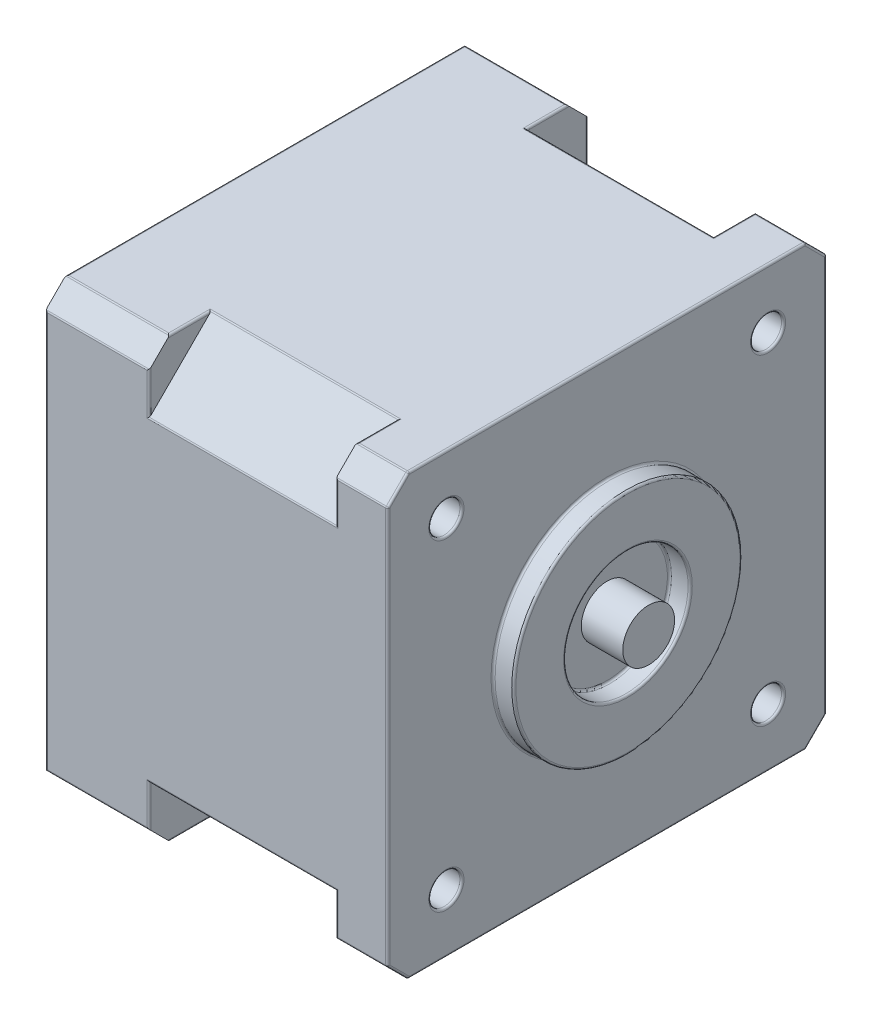
SolidWorks part; units mm, degrees
ref_plane "Front Plane" through (0, 0, 0) normal (0, 0, 1) x (1, 0, 0)
ref_plane "Top Plane" through (0, 0, 0) normal (0, 1, 0) x (1, 0, 0)
ref_plane "Right Plane" through (0, 0, 0) normal (1, 0, 0) x (0, 0, -1)
ref_plane "Plane1" through (16.5, 0, 0) normal (1, 0, 0) x (0, 0, -1)
sketch "Sketch1" plane through (16.5, 0, 0) normal (1, 0, 0) x (0, 0, -1)
  line L0 (-21.15, 19.15) -> (-21.15, -19.15)
  line L1 (-21.15, -19.15) -> (-19.15, -21.15)
  line L2 (-19.15, -21.15) -> (19.15, -21.15)
  line L3 (19.15, -21.15) -> (21.15, -19.15)
  line L4 (21.15, -19.15) -> (21.15, 19.15)
  line L5 (21.15, 19.15) -> (19.15, 21.15)
  line L6 (19.15, 21.15) -> (-19.15, 21.15)
  line L7 (-19.15, 21.15) -> (-21.15, 19.15)
extrude "Boss-Extrude1" add sketch "Sketch1" against normal blind 5
sketch "Sketch2" plane through (11.5, 0, 0) normal (-1, 0, 0) x (0, 0, 1)
  line L0 (-15.15, 21.15) -> (15.15, 21.15)
  line L1 (15.15, 21.15) -> (21.15, 15.15)
  line L2 (21.15, 15.15) -> (21.15, -15.15)
  line L3 (21.15, -15.15) -> (15.15, -21.15)
  line L4 (15.15, -21.15) -> (-15.15, -21.15)
  line L5 (-15.15, -21.15) -> (-21.15, -15.15)
  line L6 (-21.15, -15.15) -> (-21.15, 15.15)
  line L7 (-21.15, 15.15) -> (-15.15, 21.15)
extrude "Boss-Extrude2" add sketch "Sketch2" along normal blind 18
sketch "Sketch3" plane through (-6.5, 0, 0) normal (-1, 0, 0) x (0, 0, 1)
  line L0 (-19.15, -21.15) -> (-21.15, -19.15)
  line L1 (-21.15, -19.15) -> (-21.15, 19.15)
  line L2 (-21.15, 19.15) -> (-19.15, 21.15)
  line L3 (-19.15, 21.15) -> (19.15, 21.15)
  line L4 (19.15, 21.15) -> (21.15, 19.15)
  line L5 (21.15, 19.15) -> (21.15, -19.15)
  line L6 (21.15, -19.15) -> (19.15, -21.15)
  line L7 (19.15, -21.15) -> (-19.15, -21.15)
extrude "Boss-Extrude3" add sketch "Sketch3" along normal blind 10
sketch "Sketch4" plane through (0, -21.15, 0) normal (0, -1, 0) x (1, 0, 0)
  line L0 (-9.5, -5) -> (-14.5, -5)
  line L1 (-14.5, -5) -> (-14.5, 5)
  line L2 (-14.5, 5) -> (-9.5, 5)
  arc A0 (-9.5, 5) -> (-9.5, -5) centre (-9.5, 0) cw
extrude "Boss-Extrude4" add sketch "Sketch4" along normal blind 2
sketch "Sketch5" plane through (16.5, 0, 0) normal (1, 0, 0) x (0, 0, -1)
  circle A0 centre (0, 0) radius 11
extrude "Boss-Extrude5" add sketch "Sketch5" along normal blind 2
hole_wizard "Ø12.0 (12) Diameter Hole1" positions "Sketch7" profile "Sketch6" hole size "Ø12.0" standard "ANSI Metric"
sketch "Sketch7" plane through (18.5, 0, 0) normal (1, 0, 0) x (0, 0, -1)
  point P0 (0, 0)
sketch "Sketch6" plane through (18.5, 0, 0) normal (0, 1, 0) x (0, 0, -1)
  line L0 (0, 0) -> (0, 2)
  line L1 (0, 2) -> (6, 2)
  line L2 (6, 2) -> (6, 0)
  line L5 (6, 0) -> (0, 0)
  line L10 (0, 2) -> (-6, 2) construction
  line L11 (0, -6.35) -> (0, 107.95) construction
  dimension "孔直径" = 12
  dimension "孔深度" = 2
  dimension "导头角度" = 180
ref_plane "Plane2" through (0, 0, -4) normal (0, 0, 1) x (1, 0, 0)
sketch "Sketch8" plane through (0, 0, -4) normal (0, 0, 1) x (1, 0, 0)
  line L0 (-8.75, -23.15) -> (-9.5, -23.15)
  line L1 (-9.5, -23.15) -> (-9.5, -31.15)
  line L2 (-9.5, -31.15) -> (-8.75, -31.15)
  line L3 (-8.75, -31.15) -> (-8.75, -23.15)
  line L4 (-9.5, -23.15) -> (-9.5, -31.15) construction
revolve "Revolve1" add sketch "Sketch8" angle 360 about L4
ref_plane "Plane3" through (0, 0, -2) normal (0, 0, 1) x (1, 0, 0)
sketch "Sketch9" plane through (0, 0, -2) normal (0, 0, 1) x (1, 0, 0)
  line L0 (-8.75, -23.15) -> (-9.5, -23.15)
  line L1 (-9.5, -23.15) -> (-9.5, -31.15)
  line L2 (-9.5, -31.15) -> (-8.75, -31.15)
  line L3 (-8.75, -31.15) -> (-8.75, -23.15)
  line L4 (-9.5, -23.15) -> (-9.5, -31.15) construction
revolve "Revolve2" add sketch "Sketch9" angle 360 about L4
ref_plane "Plane4" through (0, 0, 4) normal (0, 0, 1) x (1, 0, 0)
sketch "Sketch10" plane through (0, 0, 4) normal (0, 0, 1) x (1, 0, 0)
  line L0 (-8.75, -23.15) -> (-9.5, -23.15)
  line L1 (-9.5, -23.15) -> (-9.5, -31.15)
  line L2 (-9.5, -31.15) -> (-8.75, -31.15)
  line L3 (-8.75, -31.15) -> (-8.75, -23.15)
  line L4 (-9.5, -23.15) -> (-9.5, -31.15) construction
revolve "Revolve3" add sketch "Sketch10" angle 360 about L4
ref_plane "Plane5" through (0, 0, 2) normal (0, 0, 1) x (1, 0, 0)
sketch "Sketch11" plane through (0, 0, 2) normal (0, 0, 1) x (1, 0, 0)
  line L0 (-8.75, -23.15) -> (-9.5, -23.15)
  line L1 (-9.5, -23.15) -> (-9.5, -31.15)
  line L2 (-9.5, -31.15) -> (-8.75, -31.15)
  line L3 (-8.75, -31.15) -> (-8.75, -23.15)
  line L4 (-9.5, -23.15) -> (-9.5, -31.15) construction
revolve "Revolve4" add sketch "Sketch11" angle 360 about L4
sketch "Sketch12" plane through (0, 0, 0) normal (0, 0, 1) x (1, 0, 0)
  line L0 (-8.75, -23.15) -> (-9.5, -23.15)
  line L1 (-9.5, -23.15) -> (-9.5, -31.15)
  line L2 (-9.5, -31.15) -> (-8.75, -31.15)
  line L3 (-8.75, -31.15) -> (-8.75, -23.15)
  line L4 (-9.5, -23.15) -> (-9.5, -31.15) construction
revolve "Revolve5" add sketch "Sketch12" angle 360 about L4
sketch "Sketch13" plane through (0, 0, 0) normal (0, 0, 1) x (1, 0, 0)
  line L0 (16.5, 2.5) -> (16.5, 0)
  line L1 (16.5, 0) -> (42.5, 0)
  line L2 (42.5, 0) -> (42.5, 2.5)
  line L3 (42.5, 2.5) -> (16.5, 2.5)
  line L4 (16.5, 0) -> (42.5, 0) construction
revolve "Revolve6" add sketch "Sketch13" angle 360 about L4
hole_wizard "Ø3.0 (3) Diameter Hole1" positions "Sketch15" profile "Sketch14" hole size "Ø3.0" standard "ANSI Metric"
sketch "Sketch15" plane through (16.5, 0, 0) normal (1, 0, 0) x (0, 0, -1)
  point P0 (-15.5, 15.5)
  point P1 (15.5, -15.5)
  point P2 (15.5, 15.5)
  point P3 (-15.5, -15.5)
sketch "Sketch14" plane through (16.5, 15.5, 15.5) normal (0, 1, 0) x (0, 0, -1)
  line L0 (0, 0) -> (0, 4.5)
  line L1 (0, 4.5) -> (1.5, 4.5)
  line L2 (1.5, 4.5) -> (1.5, 0)
  line L5 (1.5, 0) -> (0, 0)
  line L10 (0, 4.5) -> (-1.5, 4.5) construction
  line L11 (0, -6.35) -> (0, 107.95) construction
  dimension "孔直径" = 3
  dimension "孔深度" = 4.5
  dimension "导头角度" = 180
fillet "Fillet1" radius 0.2 69 edges at (-16.5, 21.15, 0) (-11.5, 21.15, -19.15) (-11.5, 21.15, 19.15) (-6.5, 21.15, -17.15) (-11.5, 19.15, -21.15) (-16.5, 0, -21.15) (-16.5, 0, 21.15) (-6.5, 21.15, 17.15) (-11.5, 19.15, 21.15) (2.5, 21.15, -15.15) (-6.5, 17.15, -21.15) (-11.5, -19.15, -21.15) (-11.5, -19.15, 21.15) (2.5, 21.15, 15.15) (-6.5, 17.15, 21.15) (11.5, 21.15, -17.15) (2.5, 15.15, -21.15) (-6.5, -17.15, -21.15) (-6.5, -17.15, 21.15) (11.5, 21.15, 17.15) (2.5, 15.15, 21.15) (14, 21.15, -19.15) (11.5, 17.15, -21.15) (2.5, -15.15, -21.15) (2.5, -15.15, 21.15) (14, 21.15, 19.15) (16.5, 21.15, 0) (11.5, 17.15, 21.15) (2.5, -21.15, -15.15) (16.5, 20.15, -20.15) (14, 19.15, -21.15) (11.5, -17.15, -21.15) (11.5, -17.15, 21.15) (16.5, 20.15, 20.15) (14, 19.15, 21.15) (11.5, -21.15, -17.15) (16.5, 0, -21.15) (14, -19.15, -21.15) (14, -19.15, 21.15) (16.5, 0, 21.15) (14, -21.15, -19.15) (16.5, -20.15, -20.15) (16.5, -20.15, 20.15) (16.5, -21.15, 0) (14, -21.15, 19.15) (11.5, -21.15, 17.15) (2.5, -21.15, 15.15) (-6.5, -21.15, 17.15) (-11.5, -21.15, 19.15) (-16.5, -21.15, 0) (-11.5, -21.15, -19.15) (16.5, 0, -6) (18.5, 0, -6) (18.5, 0, -11) (-9.5, -31.15, -0.75) (-9.5, -31.15, 1.25) (-9.5, -31.15, 3.25) (-9.5, -31.15, -2.75) (-9.5, -31.15, -4.75) (16.5, 0, -11) (16.5, 15.5, 14) (16.5, -15.5, -17) (16.5, 15.5, -17) (16.5, -15.5, 14) (42.5, 0, -2.5) (-14.5, -23.15, 0) (-12, -23.15, 5) (-12, -23.15, -5) (-4.5, -23.15, 0)
sketch "Sketch16" plane through (42.5, 0, 0) normal (1, 0, 0) x (0, 0, -1)
  circle A0 centre (0, 0) radius 3.0974
extrude "Cut-Extrude1" cut sketch "Sketch16" against normal blind 22
